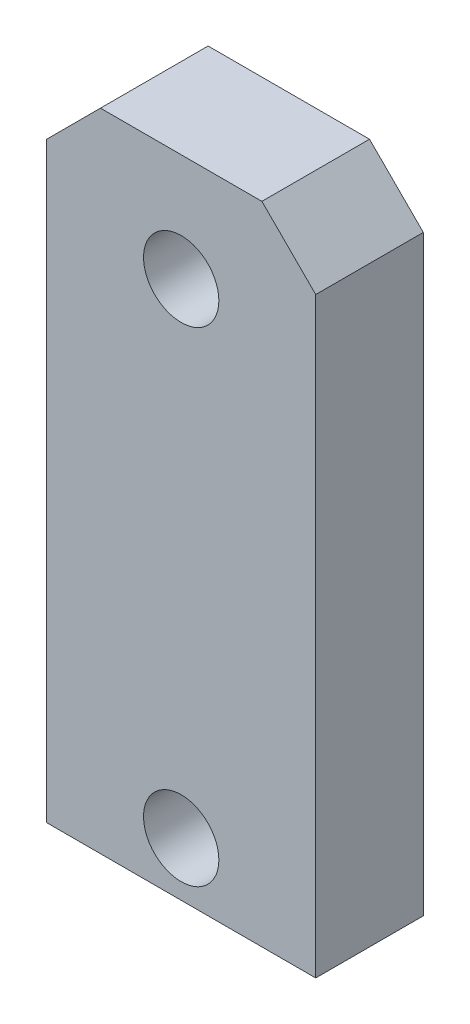
SolidWorks part; units mm, degrees
material "1023 Carbon Steel Plate (SS)"
ref_plane "Front Plane" through (0, 0, 0) normal (0, 0, 1) x (1, 0, 0)
ref_plane "Top Plane" through (0, 0, 0) normal (0, 1, 0) x (1, 0, 0)
ref_plane "Right Plane" through (0, 0, 0) normal (1, 0, 0) x (0, 0, -1)
sketch "Sketch1" plane through (0, 0, 0) normal (0, 0, 1) x (1, 0, 0)
  line L1 (12.5, 30) -> (-12.5, 30)
  line L2 (12.5, 30) -> (12.5, -30)
  line L3 (12.5, -30) -> (-12.5, -30)
  line L4 (-12.5, 30) -> (-12.5, -30)
  line L5 (12.5, 30) -> (-12.5, -30) construction
  line L6 (12.5, -30) -> (-12.5, 30) construction
  point P0 (0, 0)
  dimension "D1" = 25
  dimension "D2" = 60
extrude "Boss-Extrude1" add sketch "Sketch1" along normal blind 10
sketch "Sketch2" plane through (0, 0, 10) normal (0, 0, 1) x (1, 0, 0)
  line L0 (-12.5, -30) -> (12.5, -30) construction
  line L1 (12.5, 30) -> (-12.5, 30) construction
  circle A0 centre (0, 20) radius 3.5
  circle A1 centre (0, -25) radius 3.5
  dimension "D2" = 7
  dimension "D3" = 7
  dimension "D1" = 5
  dimension "D4" = 10
extrude "Cut-Extrude1" cut sketch "Sketch2" against normal blind 10
chamfer "Chamfer1" distance 5 angle 45 2 edges at (12.5, 30, 5) (-12.5, 30, 5)
